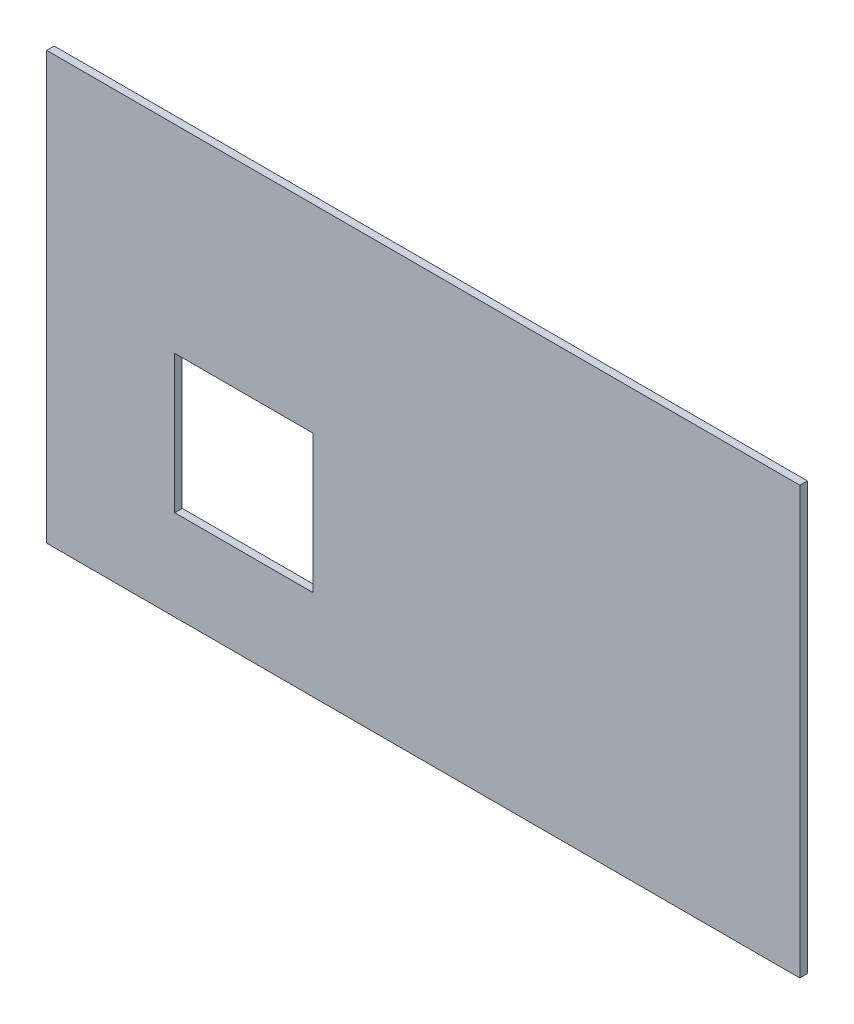
from build123d import *

# Parameters (mm, degrees)
SKETCH1_W           = 300
SKETCH1_H           = 170
BOSS_EXTRUDE1_DEPTH = 3
SKETCH2_W           = 55
SKETCH2_H           = 55
CUT_EXTRUDE2_DEPTH  = 40.5


with BuildPart() as part:
    # Sketch1 → Boss-Extrude1 (new body)
    with BuildSketch(Plane.XY):
        with Locations((-20, 0)):
            Rectangle(SKETCH1_W, SKETCH1_H)
    extrude(amount=BOSS_EXTRUDE1_DEPTH)

    # Sketch2 → Cut-Extrude2 (cut)
    with BuildSketch(Plane(origin=(0, 0, 0), x_dir=(-1, 0, 0), z_dir=(0, 0, -1))):
        with Locations((91.5, -21.5)):
            Rectangle(SKETCH2_W, SKETCH2_H)
    extrude(amount=-CUT_EXTRUDE2_DEPTH, mode=Mode.SUBTRACT)


solid = part.part
